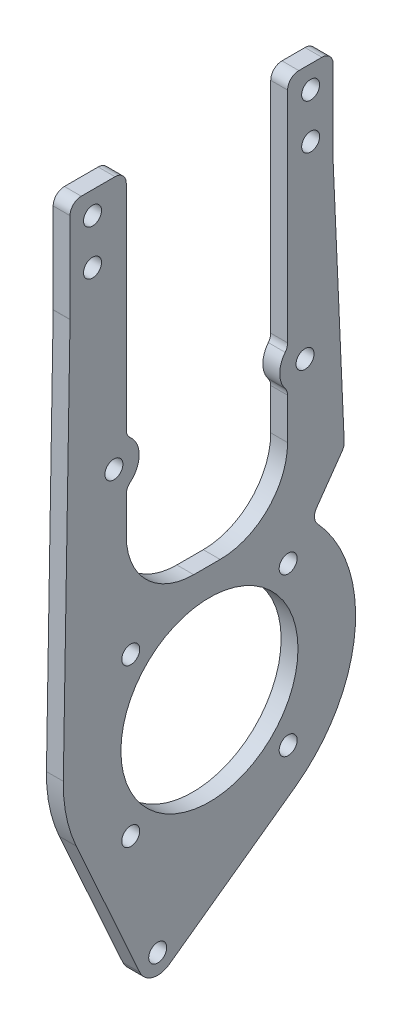
SolidWorks part; units mm, degrees
material "Thornel Mat VMA"
ref_plane "前视基准面" through (0, 0, 0) normal (0, 0, 1) x (1, 0, 0)
ref_plane "上视基准面" through (0, 0, 0) normal (0, 1, 0) x (1, 0, 0)
ref_plane "右视基准面" through (0, 0, 0) normal (1, 0, 0) x (0, 0, -1)
other "Configuration Table"
sketch "草图1" plane through (0, 0, 0) normal (1, 0, 0) x (0, 0, -1)
  line L0 (0, 0) -> (15.75, 0) construction
  line L1 (0, 0) -> (14.0007, 14.0007) construction
  line L2 (0, 0) -> (0, 16.4) construction
  line L3 (0, 16.4) -> (27.4, 16.4) construction
  line L4 (0, 0) -> (27.4, 16.4) construction
  line L5 (0, 0) -> (18.093, 18.672) construction
  line L6 (18.093, 18.672) -> (24, 27.0775)
  line L10 (0, 0) -> (-20.8, 0) construction
  line L11 (-20.8, 0) -> (-20.8, 84.9809) construction
  line L12 (-24.8, 70.9809) -> (-25.9963, 0.4409)
  line L15 (22, 88.9809) -> (-24.8, 88.9809)
  line L16 (-24.8, 70.9809) -> (-24.8, 88.9809)
  line L17 (-20.8, 84.9809) -> (18, 84.9809) construction
  line L18 (18, 84.9809) -> (18, 76.9809) construction
  line L19 (22, 88.9809) -> (22, 71.9809)
  line L20 (22, 71.9809) -> (24, 27.0775)
  circle A0 centre (0, 0) radius 15.75
  circle A1 centre (14.0007, 14.0007) radius 1.6
  circle A2 centre (14.0007, -14.0007) radius 1.6
  circle A3 centre (-14.0007, -14.0007) radius 1.6
  circle A4 centre (-14.0007, 14.0007) radius 1.6
  arc A5 (-25.9963, 0.4409) -> (18.093, 18.672) centre (0, 0) ccw
  circle A6 centre (-20.8, 84.9809) radius 1.6
  circle A7 centre (-20.8, 76.9809) radius 1.6
  circle A8 centre (18, 84.9809) radius 1.6
  circle A9 centre (18, 76.9809) radius 1.6
  point P15 (0, 0)
  dimension "D1" = 31.5
  dimension "D3" = 3.2
  dimension "D9" = 52
  dimension "D14" = 3.2
  dimension "D15" = 3.2
  dimension "D16" = 8
  dimension "D21" = 3.2
  dimension "D22" = 3.2
  dimension "D23" = 8
  dimension "D2" = 45
  dimension "D4" = 19.8
  dimension "D6" = 16.4
  dimension "D7" = 27.4
  dimension "D8" = 15
  dimension "D10" = 24
  dimension "D11" = 6
  dimension "D12" = 84.9809
  dimension "D13" = 20.8
  dimension "D17" = 4
  dimension "D18" = 24
  dimension "D19" = 4
  dimension "D20" = 38.8
  dimension "D24" = 4
  dimension "D25" = 5
  dimension "D5" = 4
extrude "凸台-拉伸1" add sketch "草图1" along normal blind 3
sketch "草图2" plane through (0, 0, 0) normal (-1, 0, 0) x (0, 0, 1)
  line L0 (-19.4985, 20.672) -> (25.6532, 20.672) construction
  line L1 (-18.093, 18.672) -> (-24, 27.0775) construction
  line L2 (24.8, 70.9809) -> (25.9963, 0.4409) construction
  line L3 (-13.9, 88.9809) -> (-13.9, 20.672) construction
  line L4 (-22, 88.9809) -> (24.8, 88.9809) construction
  line L5 (14.8, 88.9809) -> (14.8, 20.672) construction
  line L7 (-13.9, 88.9809) -> (14.8, 88.9809)
  line L8 (-13.9, 88.9809) -> (-13.9, 20.672)
  line L9 (-13.9, 20.672) -> (14.8, 20.672)
  line L10 (14.8, 88.9809) -> (14.8, 20.672)
  circle A0 centre (-18, 84.9809) radius 1.6 construction
  circle A1 centre (20.8, 84.9809) radius 1.6 construction
  dimension "D1" = 2
  dimension "D2" = 4.1
  dimension "D3" = 6
extrude "切除-拉伸1" cut sketch "草图2" against normal through all
fillet "圆角1" radius 12 2 edges at (1.5, 20.672, -13.9) (1.5, 20.672, 14.8)
sketch "草图3" plane through (0, 0, 0) normal (-1, 0, 0) x (0, 0, 1)
  line L0 (-13.9, 88.9809) -> (14.8, 88.9809) construction
  line L1 (0.45, 88.9809) -> (0.45, 20.672) construction
  line L2 (-1.9, 20.672) -> (2.8, 20.672) construction
sketch "草图4" plane through (3, 0, 0) normal (1, 0, 0) x (0, 0, -1)
  line L0 (-20.8, 76.9809) -> (-17, 76.9809) construction
  line L1 (-17, 76.9809) -> (-17, 44.0007) construction
  line L2 (-17, 44.0007) -> (17, 44.0007) construction
  circle A0 centre (-17, 44.0007) radius 1.6
  circle A1 centre (17, 44.0007) radius 1.6
  circle A2 centre (-14.0007, 14.0007) radius 1.6 construction
  dimension "D3" = 3.2
  dimension "D5" = 3.2
  dimension "D2" = 30
  dimension "D1" = 3.8
  dimension "D4" = 34
extrude "切除-拉伸2" cut sketch "草图4" against normal through all
sketch "草图5" plane through (3, 0, 0) normal (1, 0, 0) x (0, 0, -1)
  line L0 (-61.0017, -44.685) -> (6.919, -27.7505) construction
  line L1 (6.919, -27.7505) -> (0, 0) construction
  line L2 (6.919, -27.7505) -> (84.5426, -8.3967) construction
  line L3 (0, 0) -> (0, -15.75) construction
  line L4 (0, 0) -> (-19.8672, -20.5731) construction
  line L5 (-19.8672, -20.5731) -> (30.4866, -69.1992) construction
  line L6 (-12.3942, -35.7844) -> (-23.705, -10.6805)
  line L7 (-7.1585, -37.1874) -> (15.1889, -21.1021)
  circle A0 centre (0, 0) radius 15.75 construction
  circle A1 centre (-9.2032, -34.3467) radius 2.5 construction
  circle A2 centre (-9.2032, -34.3467) radius 1.6
  arc A3 (-12.3942, -35.7844) -> (-7.1585, -37.1874) centre (-9.2032, -34.3467) ccw
  arc A4 (-25.9963, 0.4409) -> (18.093, 18.672) centre (0, 0) ccw construction
  arc A5 (-23.705, -10.6805) -> (15.1889, -21.1021) centre (0, 0) ccw
  circle A6 centre (-17, 44.0007) radius 4.5
  circle A7 centre (17, 44.0007) radius 4.5
  circle A8 centre (17, 44.0007) radius 1.6 construction
  circle A9 centre (-17, 44.0007) radius 1.6 construction
  circle A10 centre (17, 44.0007) radius 1.6
  circle A11 centre (-17, 44.0007) radius 1.6
  dimension "D8" = 5
  dimension "D9" = 3.2
  dimension "D10" = 7
  dimension "D11" = 52
  dimension "D12" = 9
  dimension "D1" = 28.6
  dimension "D2" = 70
  dimension "D3" = 80
  dimension "D4" = 14
  dimension "D5" = 28.6
  dimension "D6" = 70
  dimension "D7" = 44
extrude "凸台-拉伸2" add sketch "草图5" against normal up to surface (3 mm away) up to face at (0, 44.0007, 15.4)
fillet "圆角2" radius 2 12 edges at (1.5, 88.9809, -13.9) (1.5, 88.9809, -22) (1.5, 71.9809, -22) (1.5, 27.0775, -24) (1.5, 70.9809, 24.8) (1.5, 88.9809, 24.8) (1.5, 88.9809, 14.8) (1.5, 18.672, -18.093) (1.5, 47.2626, -13.9) (1.5, 40.7388, -13.9) (1.5, 40.0752, 14.8) (1.5, 47.9263, 14.8)
